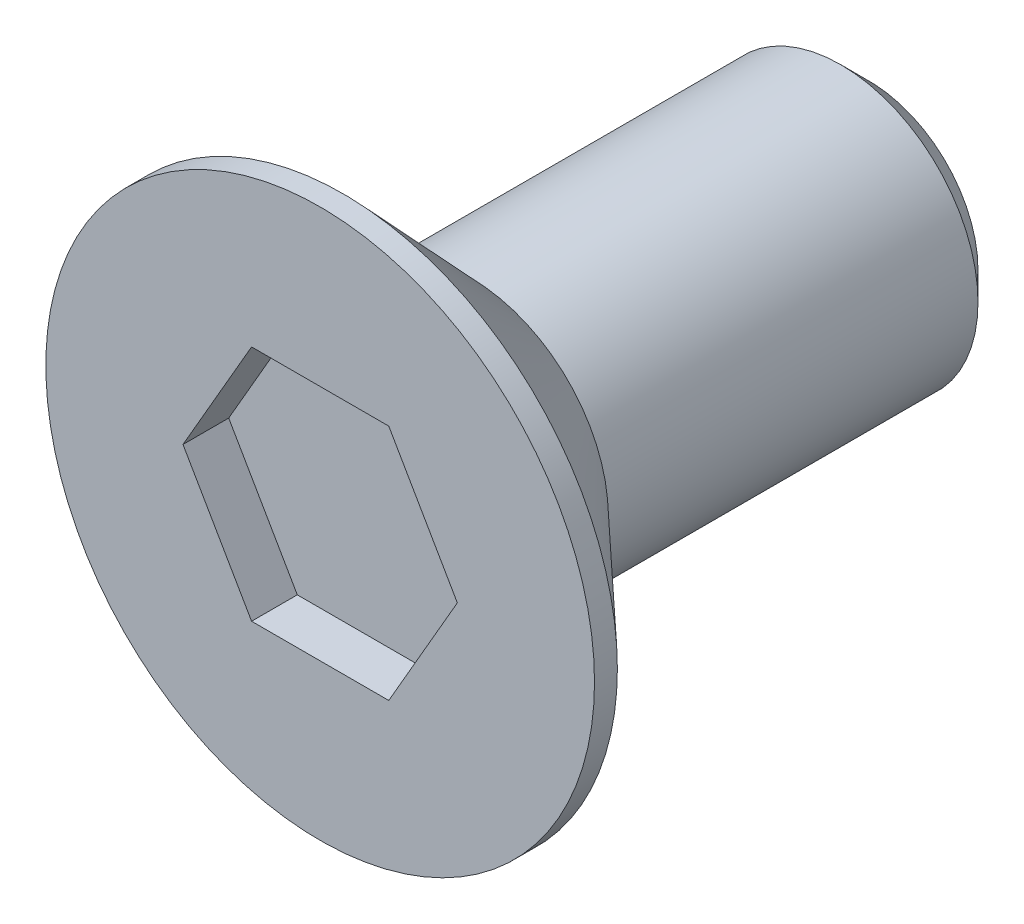
from build123d import *

# Parameters (mm, degrees)
CUT_EXTRUDE_1_DEPTH = 1
CHAMFER_1_SIZE      = 0.6135


with BuildPart() as part:
    # 草图1 → 旋转1 (revolve)
    with BuildSketch(Plane(origin=(0, 0, 0), x_dir=(1, 0, 0), z_dir=(0, 1, 0))):
        Polygon((3, 12), (0, 12), (0, 0), (6, 0), (6, 0.5), (3, 3.3), align=None)
    revolve(axis=Axis((0, 0, -12), (0, 0, 1)))

    # 草图2 → 切除-拉伸1 (cut)
    with BuildSketch(Plane.XY):
        Polygon((1.5, -2.598076211), (3, 0), (1.5, 2.598076211), (-1.5, 2.598076211), (-3, 0), (-1.5, -2.598076211), align=None)
    extrude(amount=-CUT_EXTRUDE_1_DEPTH, mode=Mode.SUBTRACT)

    # 倒角1
    chamfer_1_edges = [part.edges().sort_by_distance(p)[0] for p in [
        (-3, 0, -12),
    ]]
    chamfer(chamfer_1_edges, length=CHAMFER_1_SIZE)


solid = part.part
